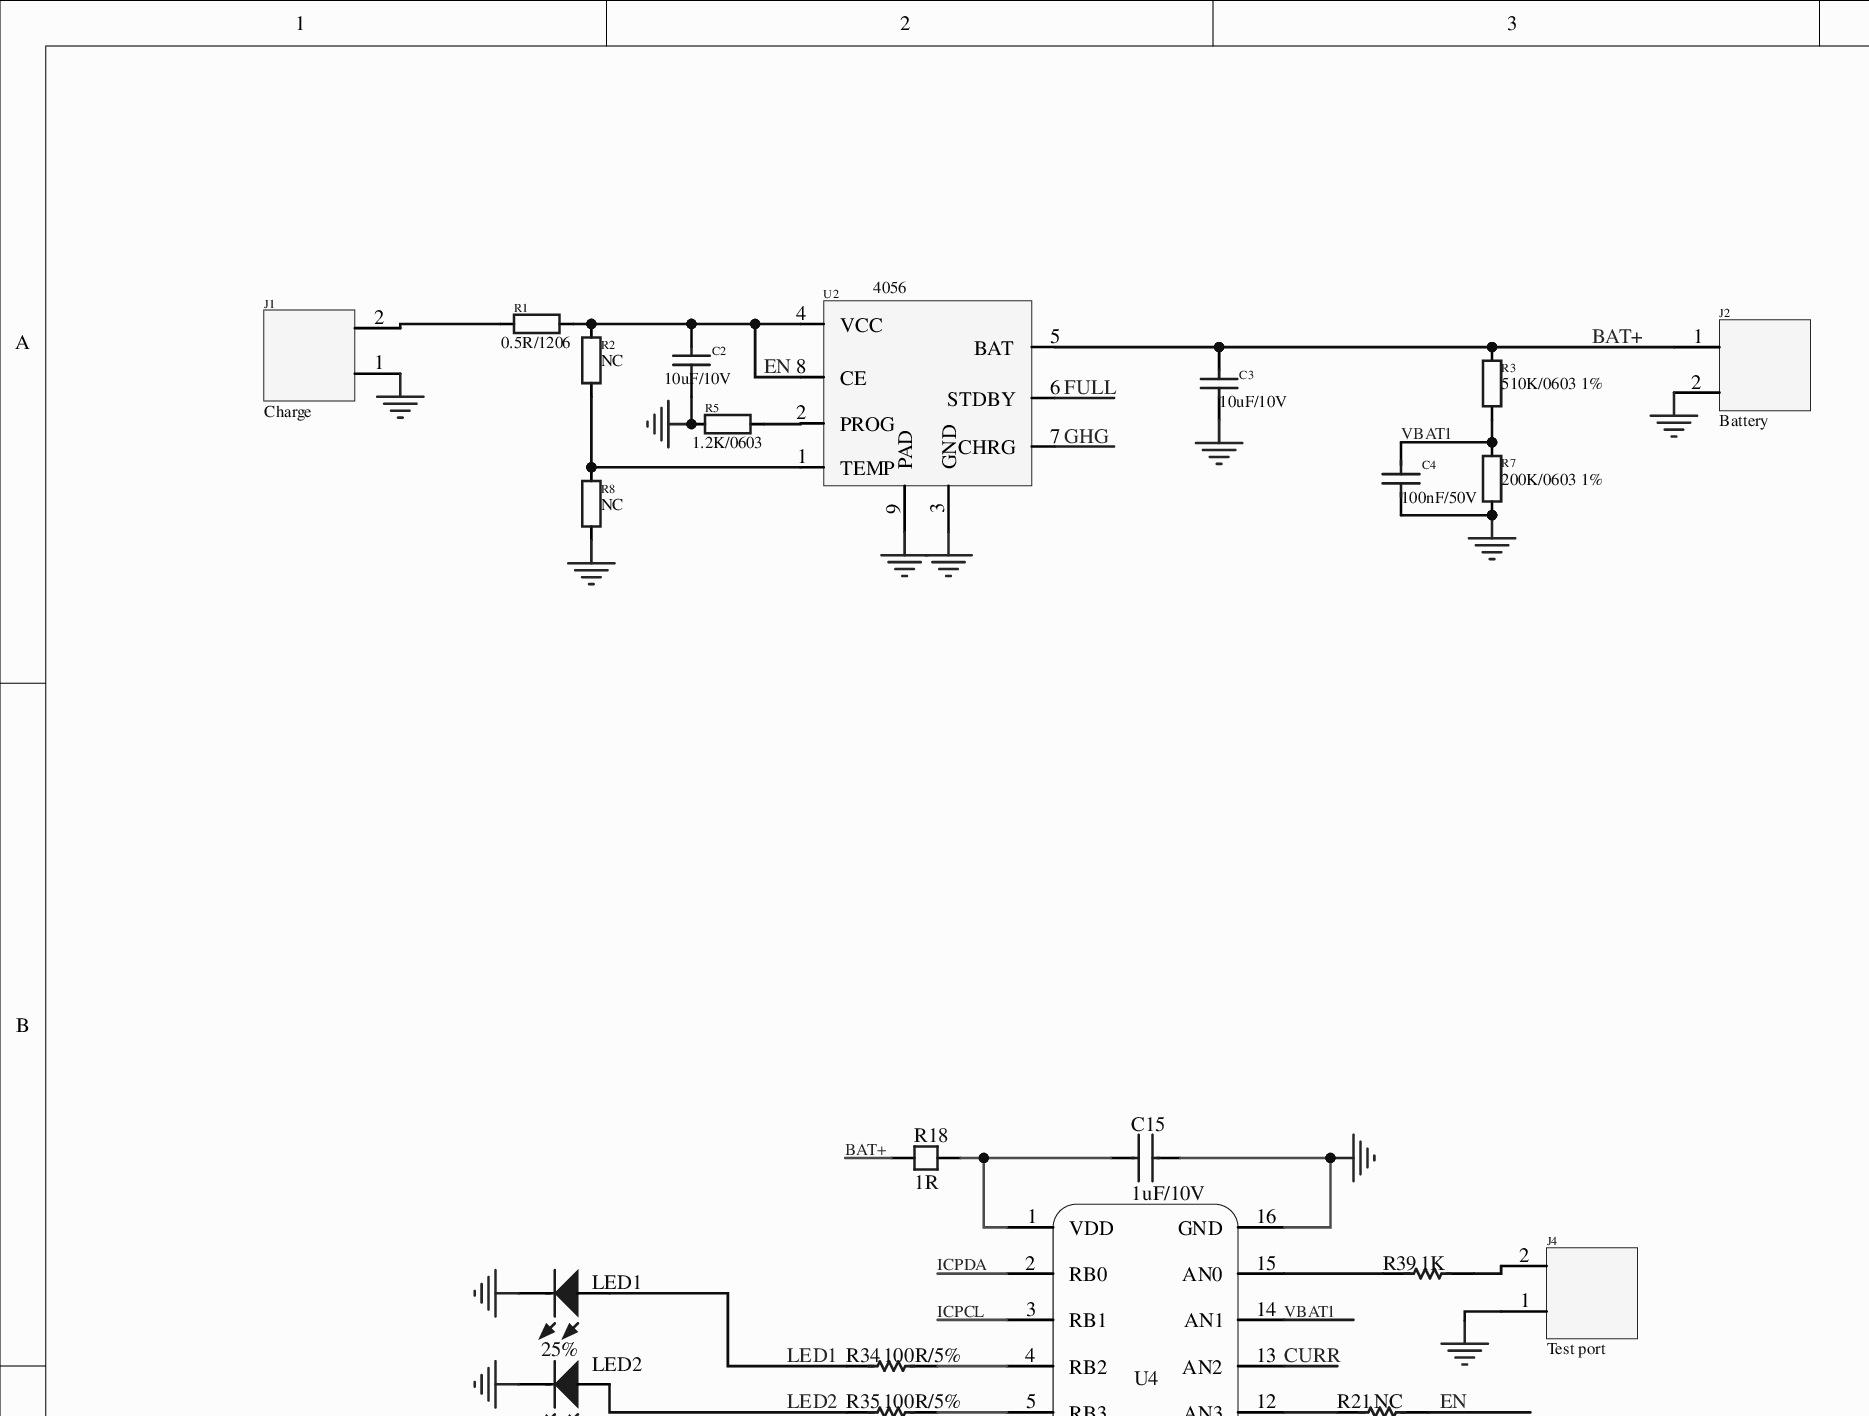
[diagram p0: MISC84244-5.SchDoc, top left]
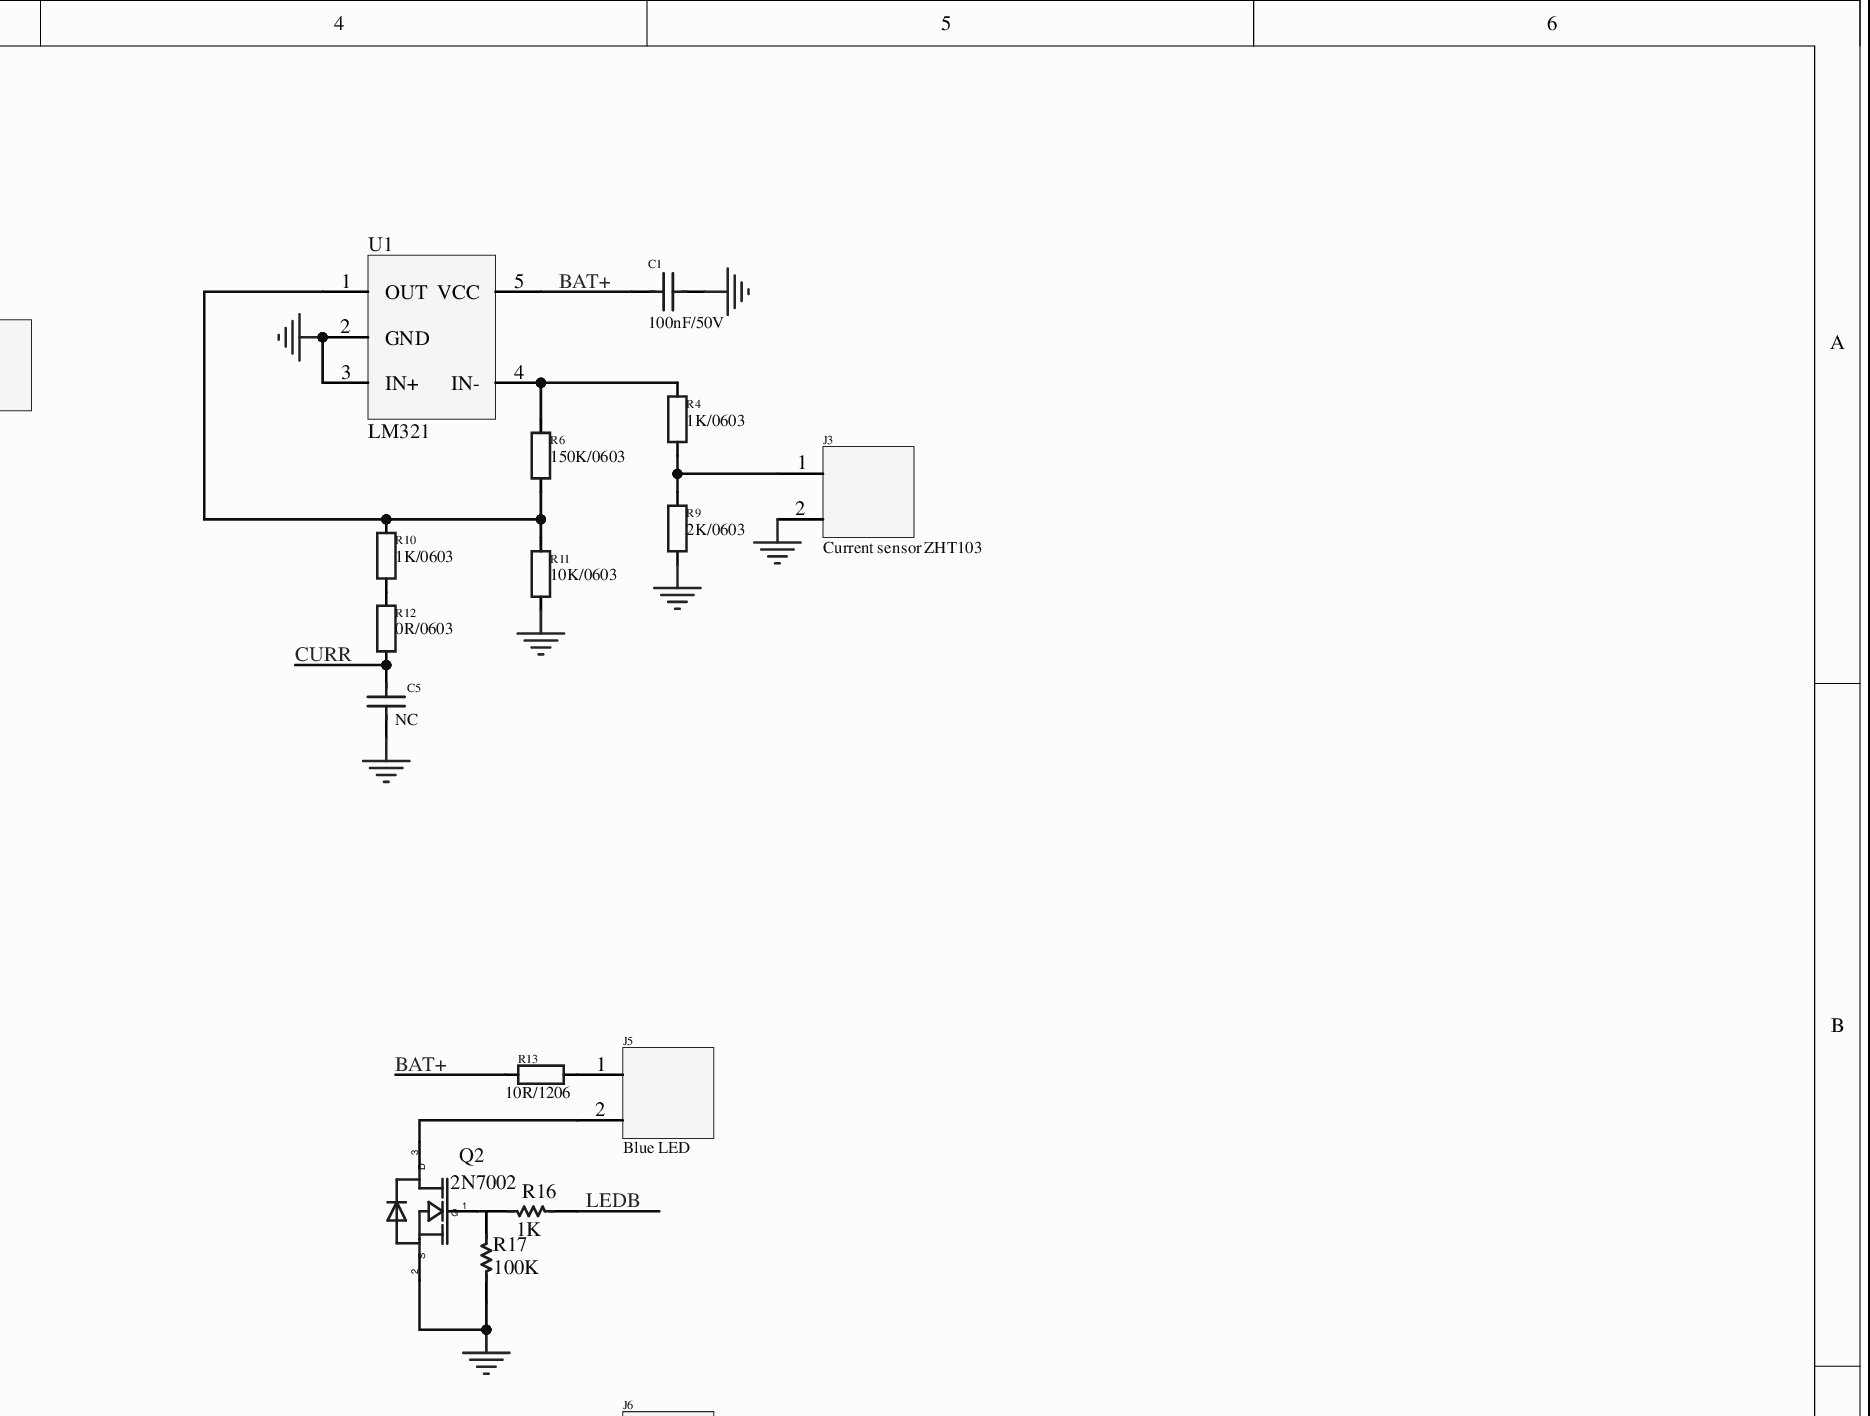
[diagram p1: MISC84244-5.SchDoc, top right]
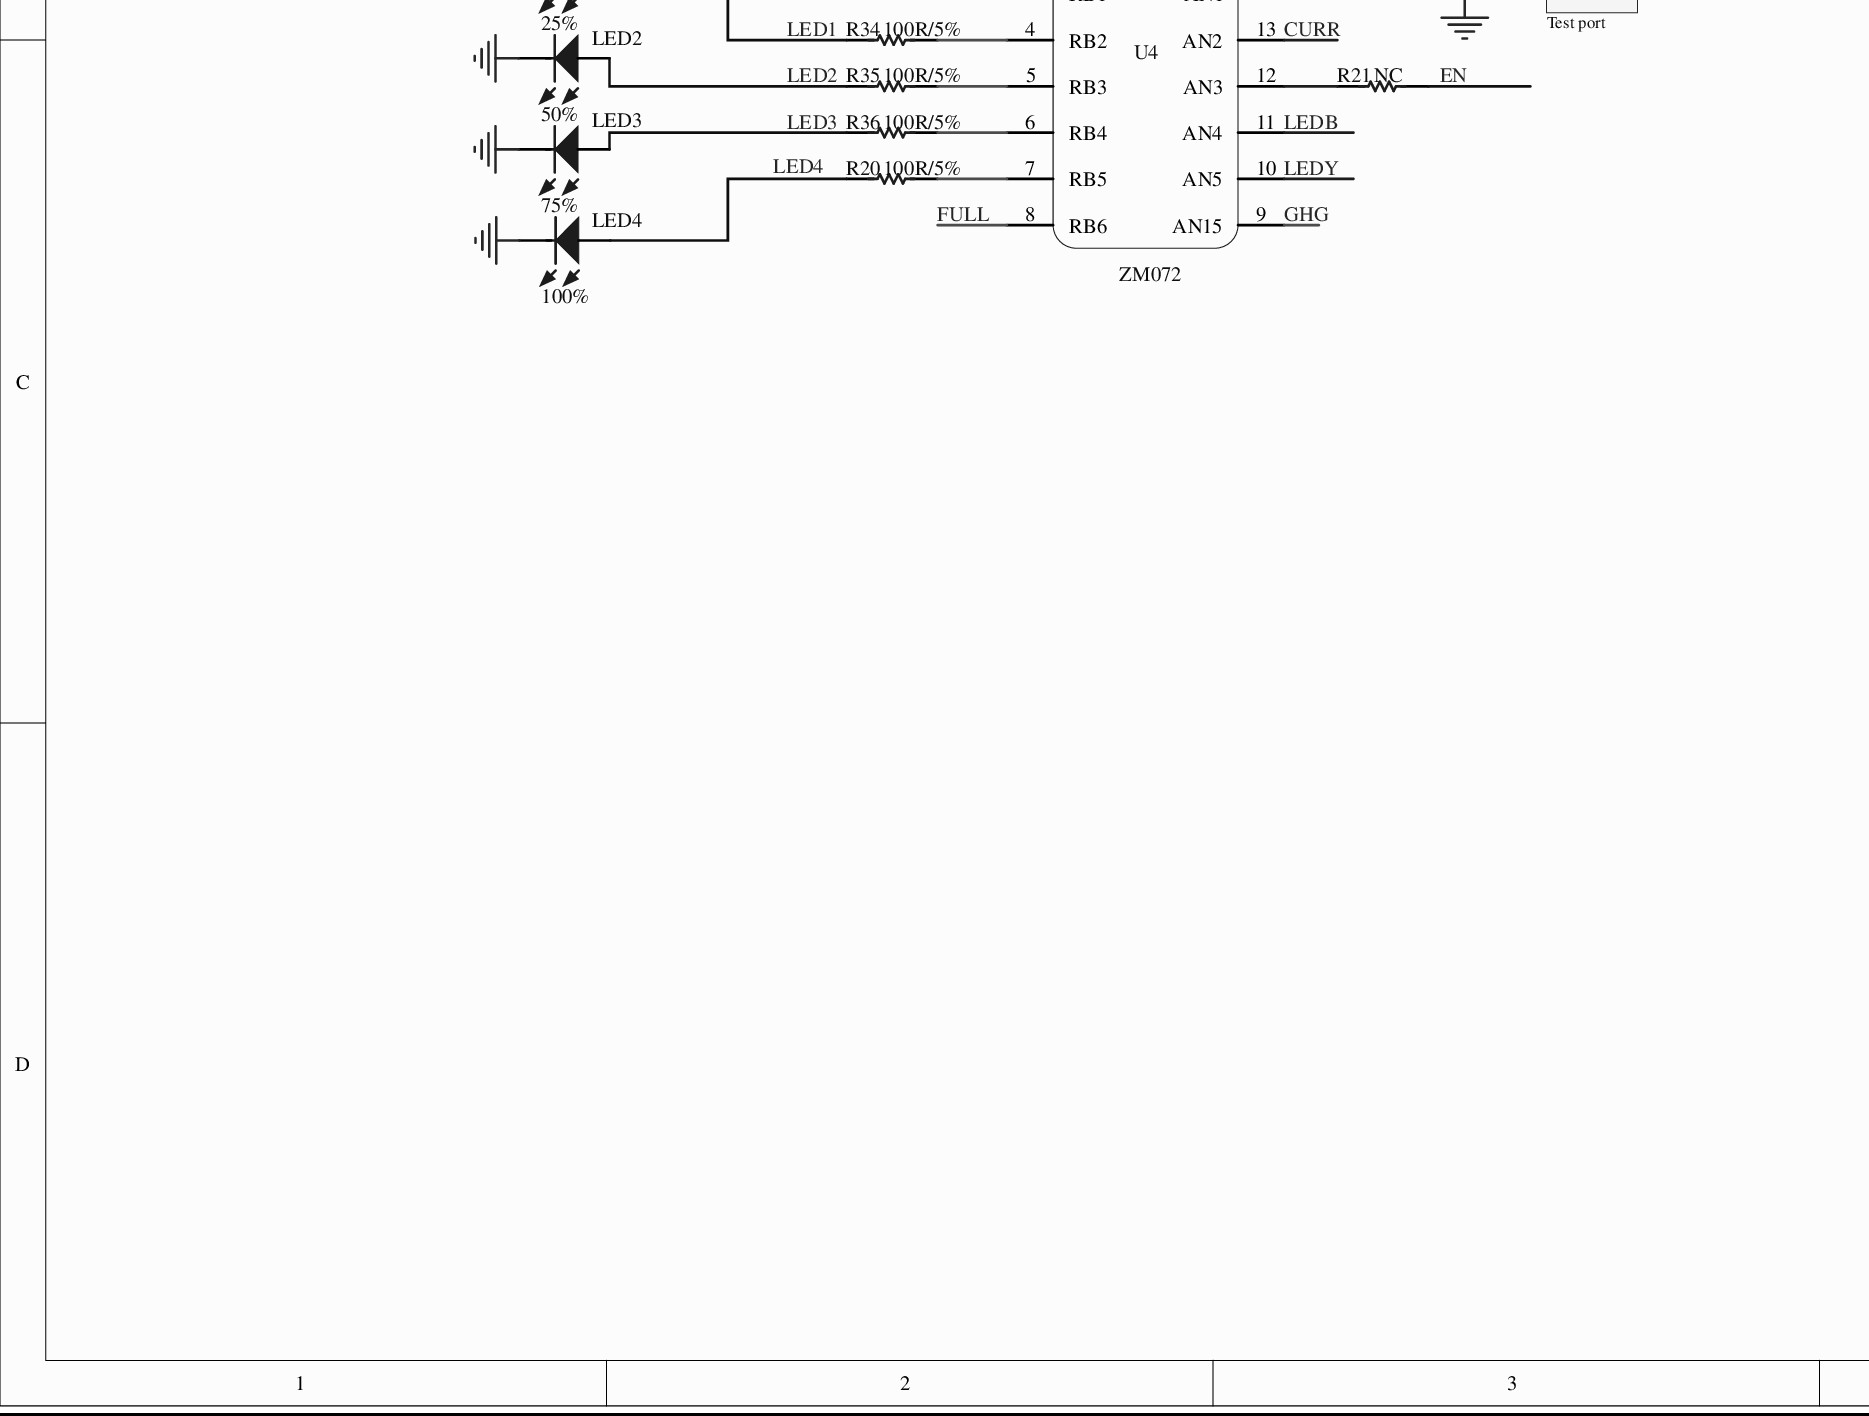
[diagram p2: MISC84244-5.SchDoc, bottom left]
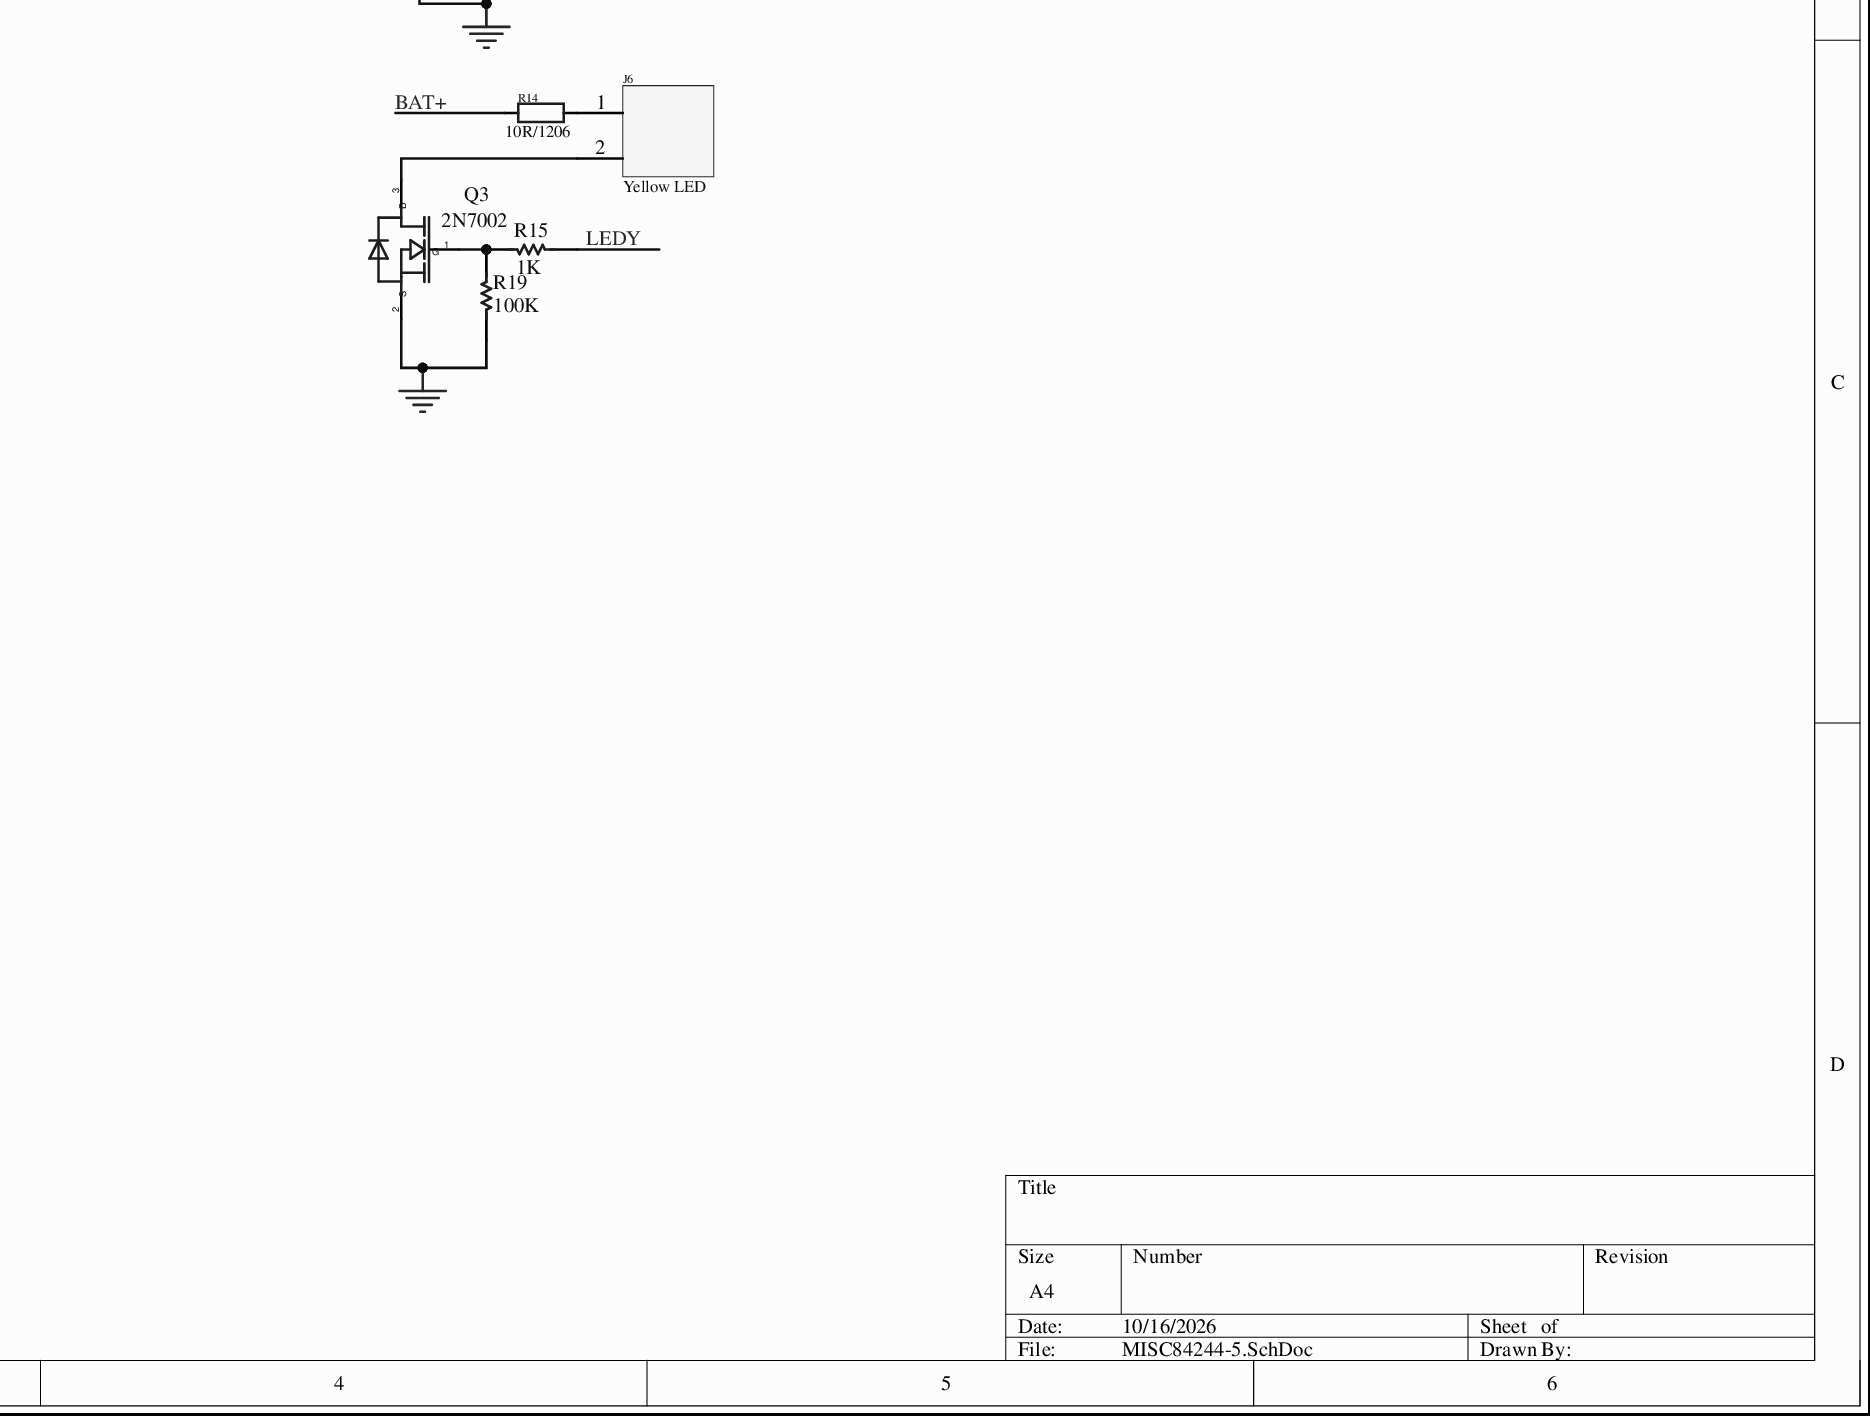
[diagram p3: MISC84244-5.SchDoc, bottom right]
# Altium project MISC84244-3.PrjPcb
1 sheet, 46 parts. Net scope: global (net labels, ports and power ports of the same name join across sheets).
Board file: MISC84244.PcbDoc

## Sheet MISC84244-5.SchDoc
size 400 x 299 mm; SheetNumber: 1; SheetTotal: 1

### Parts
C1  100nF/50V  [C0603A]
C2  10uF/10V  [C0805A]
C3  10uF/10V  [C0805A]
C4  100nF/50V  [C0603A]
C5  NC  [C0603A]
C15  1uF/10V  [C0603A]
J1  Charge  [HY2.0WT-2A/P 立贴带扣耐温260℃]
J2  Battery  [GH1.25-2PIN立贴带扣耐温260℃]
J3  Current sensor ZHT103  [IND-TH_L18.2-W10.2-P12.00-D0.9_ZHT103]
J4  Test port  [HY2.0WT-2A/P 立贴带扣耐温260℃]
J5  Blue LED  [GH1.25-2PIN立贴带扣耐温260℃]
J6  Yellow LED  [GH1.25-2PIN立贴带扣耐温260℃]
LED1  25%  [LED0603A]
LED2  50%  [LED0603A]
LED3  75%  [LED0603A]
LED4  100%  [LED0603A]
Q2  2N7002  [SOT23-3L]
Q3  2N7002  [SOT23-3L]
R1  0.5R/1206  [R1206A]
R2  NC  [R0603A]
R3  510K/0603 1%  [R0603A]
R4  1K/0603  [R0603A]
R5  1.2K/0603  [R0603A]
R6  150K/0603  [R0603A]
R7  200K/0603 1%  [R0603A]
R8  NC  [R0603A]
R9  2K/0603  [R0603A]
R10  1K/0603  [R0603A]
R11  10K/0603  [R0603A]
R12  0R/0603  [R0603A]
R13  10R/1206  [R1206A]
R14  10R/1206  [R1206A]
R15  1K  [R0603A]
R16  1K  [R0603A]
R17  100K  [R0603A]
R18  1R  [R0603A]
R19  100K  [R0603A]
R20  100R/5%  [R0603A]
R21  NC  [R0603A]
R34  100R/5%  [R0603A]
R35  100R/5%  [R0603A]
R36  100R/5%  [R0603A]
R39  1K  [R0603A]
U1  LM321  [SOT23-5A]
U2  4056  [ESOP-8L]
U4  ZM072  [SOP16L]

### Nets
GND: C1.1 C2.1 C3.1 C4.1 C5.1 C15.2 J1.1 J2.2 J3.2 J4.1 LED1.2 LED2.2 LED3.2 LED4.2 Q2.2(S) Q3.2(S) R5.1 R7.1 R8.1 R9.2 R11.2 R17.1 R19.1 U1.2(GND) U1.3(IN+) U2.3(GND) U2.9(PAD) U4.16(GND)
BAT+: C1.2 C3.2 J2.1 R3.2 R13.1 R14.1 R18.1 U1.5(VCC) U2.5(BAT)
CURR: C5.2 R12.2 U4.13(AN2)
EN: C2.2 R1.2 R2.2 R21.2 U2.4(VCC) U2.8(CE)
FULL: U2.6(STDBY) U4.8(RB6)
GHG: U2.7(CHRG) U4.9(AN15)
ICPCL: U4.3(RB1)
ICPDA: U4.2(RB0)
LED1: LED1.1 R34.1
LED2: LED2.1 R35.1
LED3: LED3.1 R36.1
LEDB: R16.2 U4.11(AN4)
LEDY: R15.2 U4.10(AN5)
VBAT1: C4.2 R3.1 R7.2 U4.14(AN1)
NetC15_1: C15.1 R18.2 U4.1(VDD)
NetJ1_2: J1.2 R1.1
NetJ3_1: J3.1 R4.2 R9.1
NetJ4_2: J4.2 R39.2
NetJ5_1: J5.1 R13.2
NetJ5_2: J5.2 Q2.3(D)
NetJ6_1: J6.1 R14.2
NetJ6_2: J6.2 Q3.3(D)
NetLED4_1: LED4.1 R20.1
NetQ2_1: Q2.1(G) R16.1 R17.2
NetQ3_1: Q3.1(G) R15.1 R19.2
NetR2_1: R2.1 R8.2 U2.1(TEMP)
NetR4_1: R4.1 R6.1 U1.4(IN-)
NetR5_2: R5.2 U2.2(PROG)
NetR6_2: R6.2 R10.1 R11.1 U1.1(OUT)
NetR10_2: R10.2 R12.1
NetR20_2: R20.2 U4.7(RB5)
NetR21_1: R21.1 U4.12(AN3)
NetR34_2: R34.2 U4.4(RB2)
NetR35_2: R35.2 U4.5(RB3)
NetR36_2: R36.2 U4.6(RB4)
NetR39_1: R39.1 U4.15(AN0)

### Notes on the sheet
- Labels drawn without touching a wire or pin: LED4

### Library data of the parts
C1 C4 C5 = Cap0603
C2 C3 = Cap0805: SMD capacitor; 规格: 0805-16V-106-X7R
C15 = CH
J1-J6 = 2PIN: DC jack right-angle 90° pitch 2.0; 物料名称: DC jack 2PIN; 封装: pitch 2.0 90° right-angle THT
LED1-LED4 = LED 白发蓝: SMD LED; 规格: 0603-diffused-ice blue
Q2 Q3 = 2N7002: SMD MOSFET
R1 R13 R14 = Res1206: SMD resistor; 规格: 0603-43.2K-1%
R2-R12 R15-R17 R19-R21 R34-R36 R39 = Res0603: SMD resistor; 规格: 0603
R18 = RH1
U2 = TP4056: Charger IC; 规格: ESOP-8; 物料名称: Charger IC 4056
U4 = MCU-TSSOP-16